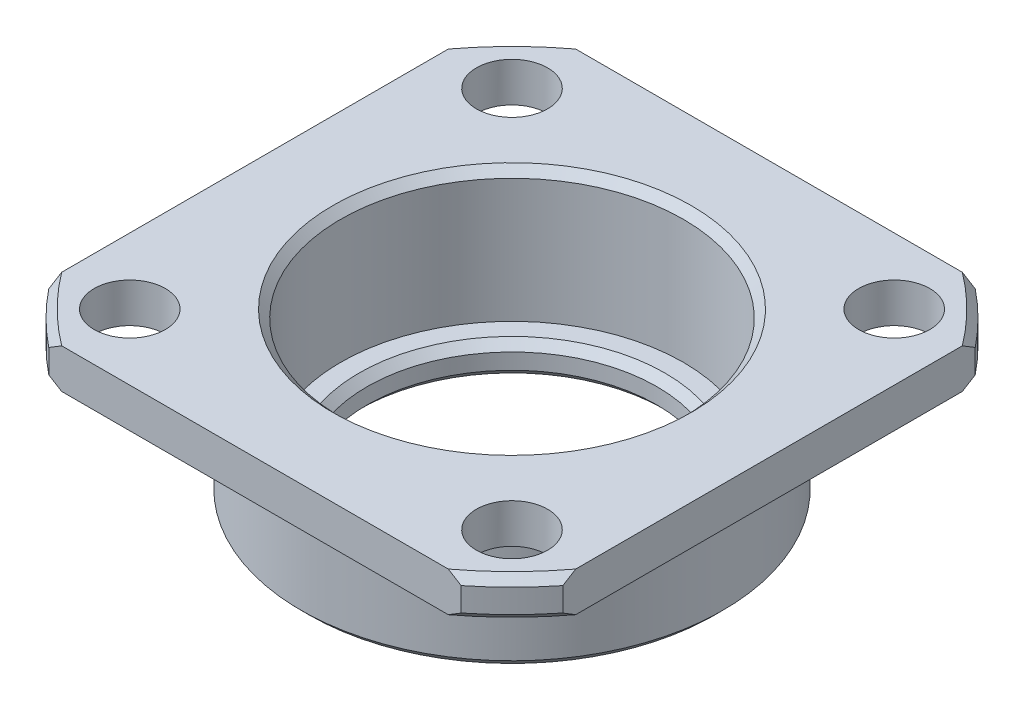
from build123d import *

# Parameters (mm, degrees)
SKETCH2_OUTSIDE_W   = 34.178
SKETCH2_OUTSIDE_H   = 34.178
SKETCH2_OUTSIDE_W_2 = 19.5
SKETCH2_OUTSIDE_H_2 = 19.5
CUT_EXTRUDE1_DEPTH  = 19.733392645
SKETCH3_R           = 1.35
CUT_EXTRUDE2_DEPTH  = 10


with BuildPart() as part:
    # Sketch1 → Revolve1 (revolve)
    with BuildSketch(Plane.XY, mode=Mode.PRIVATE) as revolve1_sk:
        Polygon((5.8, 0), (7.7, 0), (8, 0.3), (8, 4.7), (12.2, 4.7), (12.5, 5), (12.5, 5.9), (12.2, 6.2), (6.8, 6.2), (6.5, 5.9), (6.5, 1.2), (5.8, 1.2), (5.5, 0.9), (5.5, 0.3), align=None)
    revolve(revolve1_sk.sketch.rotate(Axis((0, 0, 0), (0, 1, 0)), 90), axis=Axis((0, 0, 0), (0, 1, 0)))

    # Sketch2 outside → Cut-Extrude1 (cut, through all)
    with BuildSketch(Plane(origin=(0, 6.2, 0), x_dir=(1, 0, 0), z_dir=(0, 1, 0))):
        Rectangle(SKETCH2_OUTSIDE_W, SKETCH2_OUTSIDE_H)
        Rectangle(SKETCH2_OUTSIDE_W_2, SKETCH2_OUTSIDE_H_2, mode=Mode.SUBTRACT)
    extrude(amount=-CUT_EXTRUDE1_DEPTH, mode=Mode.SUBTRACT)

    # Sketch3 → Cut-Extrude2 (cut)
    with BuildSketch(Plane(origin=(0, 6.2, 0), x_dir=(1, 0, 0), z_dir=(0, 1, 0))):
        with Locations(Location((-7.25, 7.25, 0), (0, 0, 270))):
            Circle(SKETCH3_R)
        with Locations(Location((7.25, 7.25, 0), (0, 0, 90))):
            Circle(SKETCH3_R)
        with Locations(Location((7.25, -7.25, 0), (0, 0, 270))):
            Circle(SKETCH3_R)
        with Locations(Location((-7.25, -7.25, 0), (0, 0, 90))):
            Circle(SKETCH3_R)
    extrude(amount=-CUT_EXTRUDE2_DEPTH, mode=Mode.SUBTRACT)


solid = part.part
